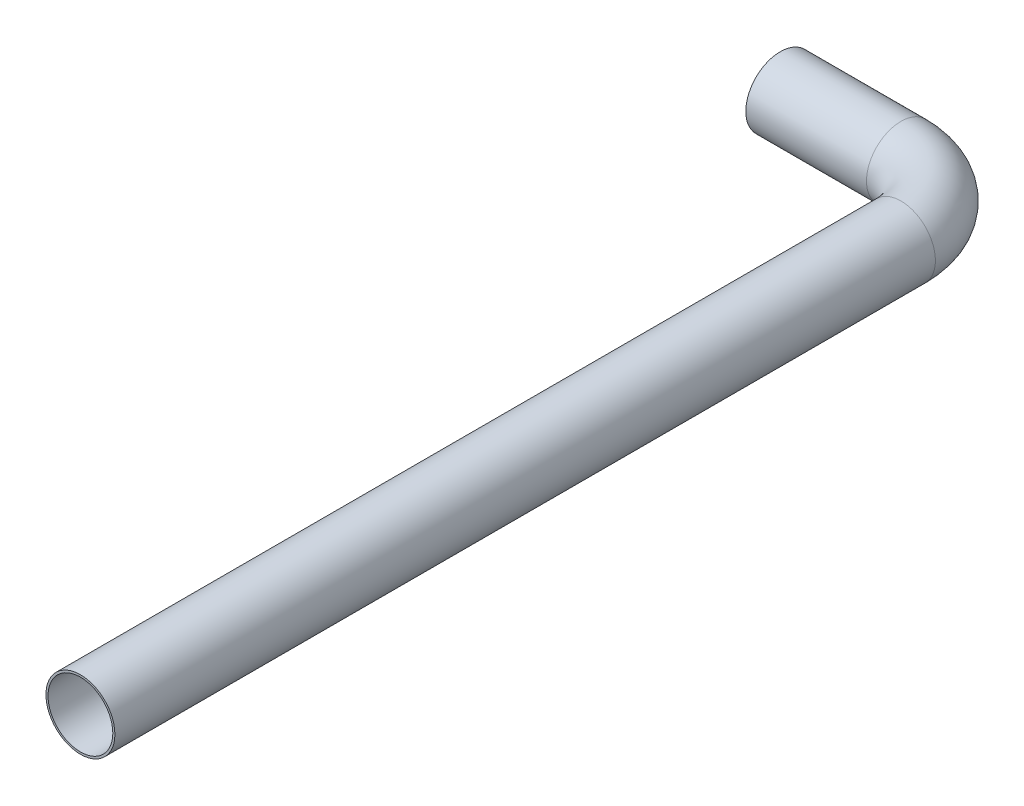
from build123d import *

# Parameters (mm, degrees)
SKETCH_1_R = 50
SHELL_1_T  = -3


with BuildPart() as part:
    # 扫描1: sweep along a path in 草图2
    with BuildLine(Plane(origin=(0, 0, 0), x_dir=(1, 0, 0), z_dir=(0, 1, 0))) as sweep_1_path:
        Line((0, 0), (0, 1190))
        ThreePointArc((0, 1190), (-29.289321881, 1260.710678119), (-100, 1290))
        Line((-100, 1290), (-275, 1290))
    # 草图1 → 扫描1 (sweep)
    with BuildSketch(Plane.XY):
        Circle(SKETCH_1_R)
    sweep(path=sweep_1_path.line)

    # 抽壳1
    shell_1_openings = [part.faces().sort_by_distance(p)[0] for p in [
        (-275, 0, -1290),
        (0, 0, 0),
    ]]
    offset(amount=SHELL_1_T, openings=shell_1_openings, kind=Kind.INTERSECTION)


solid = part.part
